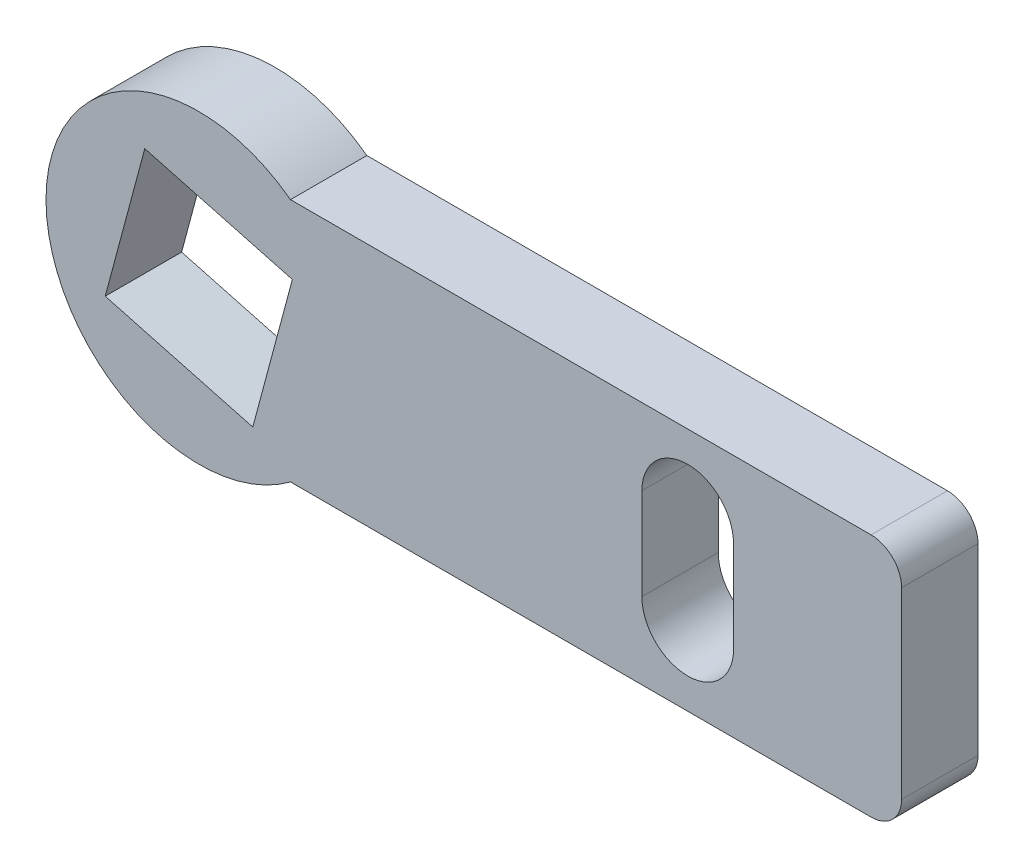
from build123d import *

# Parameters (mm, degrees)
EXTRUDE_1_DEPTH     = 1.25
CUT_EXTRUDE_1_DEPTH = 24.669600757
FILLET_1_R          = 1


with BuildPart() as part:
    # 草图1 → 凸台-拉伸1 (new, symmetric)
    with BuildSketch(Plane.XY):
        with BuildLine():
            Line((3, 4), (23, 4))
            Line((23, 4), (23, -4))
            Line((23, -4), (3, -4))
            ThreePointArc((3, -4), (-5, 0), (3, 4))
        make_face()
    extrude(amount=EXTRUDE_1_DEPTH, both=True)

    # 草图2 → 切除-拉伸1 (cut, through all)
    with BuildSketch(Plane.XY.offset(1.25)):
        Polygon((1.767766953, -3.061862178), (3.061862178, 1.767766953), (-1.767766953, 3.061862178), (-3.061862178, -1.767766953), align=None)
        with BuildLine():
            Line((14.5, -1.5), (14.5, 1.5))
            ThreePointArc((14.5, 1.5), (16, 3), (17.5, 1.5))
            Line((17.5, 1.5), (17.5, -1.5))
            ThreePointArc((17.5, -1.5), (16, -3), (14.5, -1.5))
        make_face()
    extrude(amount=-CUT_EXTRUDE_1_DEPTH, mode=Mode.SUBTRACT)

    # 圆角1
    fillet_1_edges = [part.edges().sort_by_distance(p)[0] for p in [
        (23, 4, 0),
        (23, -4, 0),
    ]]
    fillet(fillet_1_edges, radius=FILLET_1_R)


solid = part.part
